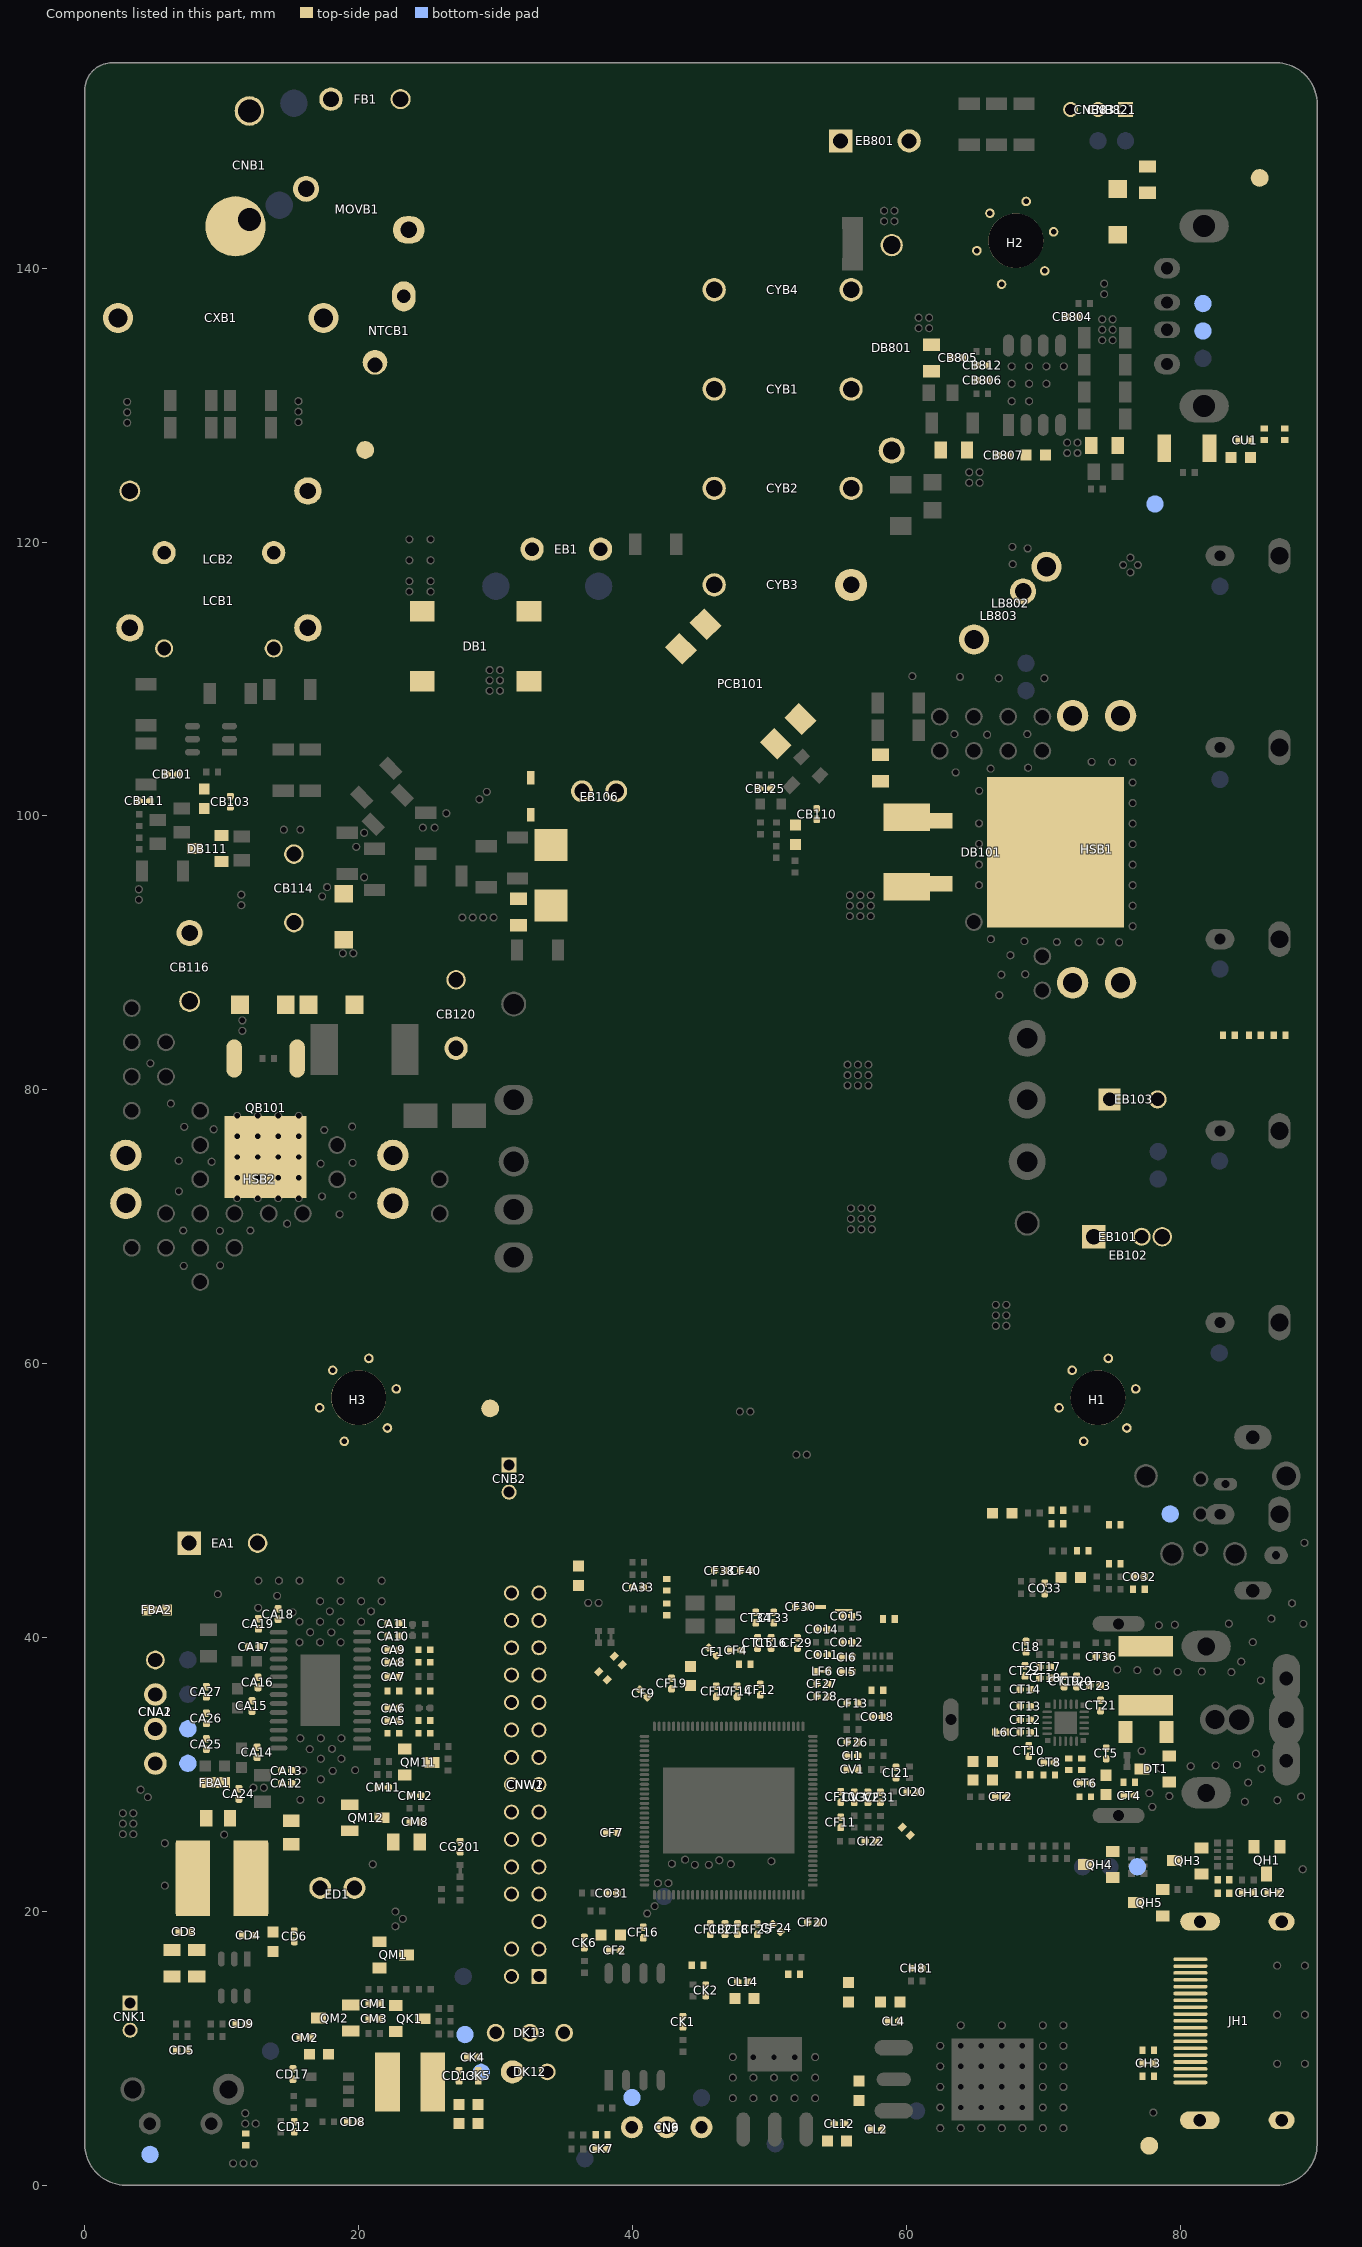
[diagram p0: the components of this part, seen from the top]
# Altium PCB MISC116569.PcbDoc (part 2 of 15)
Units mm, origin at the board's own origin, x right, y up, seen from the top; angles counter-clockwise.
Board outline 90 x 155 mm, 2 copper layers (TopLayer, BottomLayer), stack 1.571 mm thick; 527 components, 277 nets, 2450 pads, 649 vias.

## Components (designator, comment, footprint, x,y, rotation, side; value= is the part's Value field where it differs from the comment) (continued)
CA5 "0.22uF-0402-X5R-±10%-16V" C0402#1 22.539,33.929 r180 top
CA6 "0.22uF-0402-X5R-±10%-16V" C0402#1 22.539,34.849 r180 top
CA7 "1uF-0402-X5R-±20%-16V" C0402#1 22.539,37.145 r180 top
CA8 "1uF-0402-X5R-±20%-16V" C0402#1 22.539,38.177 r180 top
CA9 "NC/1uF-0402-X5R-±20%-16V" C0402#1 22.539,39.107 r180 top
CA10 "0.22uF-0402-X5R-±10%-16V" C0402#1 22.539,40.101 r180 top
CA11 "0.22uF-0402-X5R-±10%-16V" C0402#1 22.539,41.018 r180 top
CA12 "NC/0.1uF-0402-X5R-±20%-16V" C0402#1 14.752,29.358 r180 top
CA13 "1000pF-0402-X7R-±10%-50V" C0402#1 14.752,30.274 r180 top
CA14 "0.22uF-0402-X5R-±10%-16V" C0402#1 12.586,31.619 r270 top
CA15 "0.22uF-0402-X5R-±10%-16V" C0402#1 12.205,34.997 r270 top
CA16 "0.22uF-0402-X5R-±10%-16V" C0402#1 12.649,36.722 r90 top
CA17 "0.22uF-0402-X5R-±10%-16V" C0402#1 12.361,39.332 r180 top
CA18 "NC/0.1uF-0402-X5R-±20%-16V" C0402#1 14.122,41.716 r270 top
CA19 "1000pF-0402-X7R-±10%-50V" C0402#1 12.675,41.002 r270 top
CA24 "2200pF-0402-X7R-±10%-50V" C0402#1 11.252,28.581 r90 top
CA25 "2200pF-0402-X7R-±10%-50V" C0402#1 8.877,32.22 r90 top
CA26 "2200pF-0402-X7R-±10%-50V" C0402#1 8.877,34.095 r90 top
CA27 "2200pF-0402-X7R-±10%-50V" C0402#1 8.878,36.039 r270 top
CA31 "NC/10uF-0603-X5R-±20%-6.3V" C0603 67,49.075 r180 top
CA32 "NC/10uF-0603-X5R-±20%-6.3V" C0603 72.001,44.375 r180 top
CA33 "NC/1uF-0402-X5R-±20%-6.3V" C0402#1 40.411,43.665 r180 top
CAUTION "CAUTION" CAUTION 30.264,127.254 r180 bottom
CB101 "100pF-0402-NPO-±5%-50V" C0402#1 6.382,103.035 r180 top
CB102 "0.1uF-0603-X7R-±10%-50V" C0603 8.725,101.244 r270 top
CB103 "1000pF-0402-X7R-±10%-50V" C0402#1 10.63,101.041 r90 top
CB109 "Ceramic capacitor,CAP MC,25V,0.22uF,±10%,X7R,0603,SMD,TP" C0603 51.887,98.633 r270 top
CB110 "NC/1000pF-0402-X7R-±10%-50V" C0402#1 53.454,100.133 r90 top
CB111 "NC/Ceramic capacitor,CAP MC,50V,100pF,±5%,NPO,0402,SMD,TP" C0402#1 4.36,101.098 r0 top
CB113 "NC/220PF-0805-NPO-±10%-200V" C0805 31.661,92.989 r90 top
CB114 "Film capacitor,CAP PE,400V,4700pF,±5%,P,5.0mm,PC,DIP,TP,Fara" CAP8*2.5-V-5 15.269,94.709 r270 top locked
CB116 "Ceramic capacitor,CAP CD,2KV,100pF,±5%,SL,IK,5.0mm,DIP,TP,Walsin" CAP6.5*5-V-5-1 7.658,88.951 r270 top locked
CB118 "1000pF-0805-NPO-±10%-200V" C0805 58.11,103.505 r90 top
CB120 "NC/Ceramic capacitor,CAP CD,1KV,4700pF,±20%,Y5U,K,5.0mm,DIP,TP,Walsin" CAP10*4.5-V-5 27.114,85.534 r90 top locked
CB125 "NC/Ceramic capacitor,CAP MC,50V,0.022uF,±10%,X7R,0402,SMD,TP" C0402#1 49.677,101.994 r0 top
CB801 "Ceramic capacitor,CAP MC,25V,1uF,±10%,X7R,0603,SMD,TP" C0603 69.456,126.362 r180 top
CB804 "4700pF-0402-X7R-±10%-50V" C0402#1 72.098,136.449 r180 top
CB805 "NC/0.1uF-0402-X7R-±10%-16V" C0402#1 63.745,133.477 r180 top
CB806 "1000pF-0402-X7R-±10%-50V" C0402#1 65.54,131.826 r180 top
CB807 "100pF-0402-NPO-±5%-50V" C0402#1 67.076,126.34 r0 top
CB808 "220PF-0805-NPO-±10%-200V" C0805 77.597,146.468 r90 top
CB809 "220PF-0805-NPO-±10%-200V" C0805 74.481,127.051 r180 top
CB810 "220PF-0805-NPO-±10%-200V" C0805 63.469,126.733 r0 top
CB811 "220PF-0805-NPO-±10%-200V" C0805 61.831,133.452 r270 top
CB812 "0.033uF-0402-X7R-±10%-16V" C0402#1 65.54,132.918 r180 top
CD1 "NC/10uF-0805-X5R-±20%-16V" C0805 8.174,16.207 r270 top
CD2 "10uF-0805-X5R-±20%-16V" C0805 6.365,16.207 r270 top
CD3 "NC/0.1uF-0402-X5R-±20%-16V" C0402#1 7.276,18.504 r0 top
CD4 "Ceramic capacitor,CAP MC,16V,0.1uF,±10%,X7R,0402,SMD,TP" C0402#1 11.92,18.25 r0 top
CD5 "NC/56pF-0402-NPO-±5%-50V" C0402#1 7.088,9.868 r180 top
CD6 "NC/0.1uF-0402-X5R-±20%-16V" C0402#1 15.299,18.174 r90 top
CD7 "10uF-0603-X5R-±20%-6.3V" C0603 13.749,17.788 r90 top
CD8 "1uF-0402-X5R-±20%-6.3V" C0402#1 19.575,4.638 r180 top
CD9 "NC/0.1uF-0402-X5R-±20%-16V" C0402#1 11.434,11.786 r180 top
CD10 "NC/10uF-0603-X5R-±20%-6.3V" C0603 38.417,18.275 r180 top
CD12 "NC/NC/3300pF-0402-X7R-±10%-50V" C0402#1 15.299,4.27 r270 top
CD13 "NC/0.1uF-0402-X5R-±20%-16V" C0402#1 27.338,7.991 r270 top
CD14 "10uF-0603-X5R-±20%-6.3V" C0603 28.729,5.197 r90 top
CD15 "10uF-0603-X5R-±20%-6.3V" C0603 27.345,5.197 r90 top
CD16 "10uF-0603-X5R-±20%-6.3V" C0603 17.102,9.563 r180 top
CD17 "NC/0.1uF-0402-X5R-±20%-16V" C0402#1 15.197,8.118 r90 top
CF1 "Ceramic capacitor,CAP MC,50V,18pF,±5%,NPO,0402,SMD,TP" C0402#1 45.846,38.965 r315 top
CF2 "Ceramic capacitor,CAP MC,16V,0.1uF,±10%,X7R,0402,SMD,TP" C0402#1 38.714,17.147 r180 top
CF3 "10uF-0603-X5R-±20%-6.3V" C0603 44.221,37.186 r270 top
CF4 "Ceramic capacitor,CAP MC,50V,18pF,±5%,NPO,0402,SMD,TP" C0402#1 47.535,39.068 r180 top
CF5 "10uF-0603-X5R-±20%-6.3V" C0603 55.761,14.099 r90 top
CF7 "Ceramic capacitor,CAP MC,16V,0.1uF,±10%,X7R,0402,SMD,TP" C0402#1 38.482,25.745 r0 top
CF8 "Ceramic capacitor,CAP MC,16V,0.1uF,±10%,X7R,0402,SMD,TP" C0402#1 47.666,18.708 r90 top
CF9 "Ceramic capacitor,CAP MC,16V,0.1uF,±10%,X7R,0402,SMD,TP" C0402#1 40.8,35.918 r315 top
CF10 "Ceramic capacitor,CAP MC,16V,0.1uF,±10%,X7R,0402,SMD,TP" C0402#1 55.207,28.355 r90 top
CF11 "Ceramic capacitor,CAP MC,16V,0.1uF,±10%,X7R,0402,SMD,TP" C0402#1 55.207,26.505 r270 top
CF12 "Ceramic capacitor,CAP MC,16V,0.1uF,±10%,X7R,0402,SMD,TP" C0402#1 49.335,36.197 r270 top
CF13 "Ceramic capacitor,CAP MC,16V,0.1uF,±10%,X7R,0402,SMD,TP" C0402#1 56.071,35.204 r180 top
CF14 "Ceramic capacitor,CAP MC,16V,0.1uF,±10%,X7R,0402,SMD,TP" C0402#1 47.638,36.067 r270 top
CF15 "10uF-0603-X5R-±20%-6.3V" C0603 36.063,44.503 r270 top
CF16 "Ceramic capacitor,CAP MC,16V,0.1uF,±10%,X7R,0402,SMD,TP" C0402#1 40.787,18.456 r90 top
CF17 "Ceramic capacitor,CAP MC,16V,0.1uF,±10%,X7R,0402,SMD,TP" C0402#1 46.114,36.067 r270 top
CF18 "Ceramic capacitor,CAP MC,16V,0.1uF,±10%,X7R,0402,SMD,TP" C0402#1 45.683,18.708 r270 top
CF19 "Ceramic capacitor,CAP MC,16V,0.1uF,±10%,X7R,0402,SMD,TP" C0402#1 42.85,36.643 r90 top
CF20 "Ceramic capacitor,CAP MC,16V,0.1uF,±10%,X7R,0402,SMD,TP" C0402#1 53.187,19.192 r180 top
CF21 "1uF-0402-X5R-±20%-6.3V" C0402#1 46.749,18.708 r270 top
CF24 "1uF-0402-X5R-±20%-6.3V" C0402#1 50.525,18.792 r315 top
CF25 "1uF-0402-X5R-±20%-6.3V" C0402#1 49.112,18.708 r270 top
CF26 "0.047uF-0402-X7R-±10%-16V" C0402#1 56.07,32.36 r0 top
CF27 "NC/0.1uF-0402-X5R-±20%-16V" C0402#1 53.868,36.614 r180 top
CF28 "1uF-0402-X5R-±20%-6.3V" C0402#1 53.868,35.7 r180 top
CF29 "NC/1000pF-0402-X7R-±10%-50V" C0402#1 52.04,39.605 r270 top
CF30 "NC/1000pF-0402-X7R-±10%-50V" C0402#1 52.294,42.23 r0 top
CF31 "0.047uF-0402-X7R-±10%-16V" C0402#1 58.102,28.334 r270 top
CF38 "NC/30pF-0402-NPO-±5%-50V" C0402#1 46.375,44.884 r0 top
CF40 "Ceramic capacitor,CAP MC,50V,0.01uF,±10%,X7R,0402,SMD,TP" C0402#1 48.274,44.884 r180 top
CG201 "NC/0.1uF-0402-X5R-±20%-16V" C0402#1 27.414,24.719 r90 top
CH1 "NC/0.1uF-0402-X5R-±20%-16V" C0402#1 84.945,21.365 r0 top
CH2 "NC/0.1uF-0402-X5R-±20%-16V" C0402#1 86.8,21.364 r0 top
CH3 "NC/Ceramic capacitor,CAP MC,50V,22pF,±5%,NPO,0402,SMD,TP" C0402#1 77.664,8.905 r180 top
CH81 "1uF-0402-X5R-±20%-6.3V" C0402#1 60.765,15.839 r180 top
CI1 "0.047uF-0402-X7R-±10%-16V" C0402#1 56.062,31.355 r0 top
CI5 "Ceramic capacitor,CAP MC,16V,0.1uF,±10%,X7R,0402,SMD,TP" C0402#1 55.646,37.506 r0 top
CI6 "Ceramic capacitor,CAP MC,16V,0.1uF,±10%,X7R,0402,SMD,TP" C0402#1 55.646,38.572 r0 top
CI18 "NC/30pF-0402-NPO-±5%-50V" C0402#1 68.745,39.332 r270 top
CI20 "NC/NC/10pF-0402-NPO-±5%-50V" C0402#1 60.446,28.727 r0 top
CI21 "NC/NC/10pF-0402-NPO-±5%-50V" C0402#1 59.245,30.137 r270 top
CI22 "NC/NC/10pF-0402-NPO-±5%-50V" C0402#1 57.387,25.133 r0 top
CK1 "NC/0.1uF-0402-X7R-±20%-16V" C0402#1 43.683,11.937 r270 top
CK2 "Ceramic capacitor,CAP MC,50V,0.01uF,±10%,X7R,0402,SMD,TP" C0402#1 45.347,14.227 r270 top
CK4 "NC/0.1uF-0402-X5R-±20%-16V" C0402#1 28.341,9.362 r0 top
CK5 "NC/0.1uF-0402-X5R-±20%-16V" C0402#1 28.735,7.991 r270 top
CK6 "NC/10pF-0402-NPO-±5%-50V" C0402#1 36.482,17.719 r270 top
CK7 "NC/Ceramic capacitor,CAP MC,16V,0.1uF,±10%,X7R,0402,SMD,TP" C0402#1 37.731,2.657 r0 top
CL1 "NC/10uF-0603-X5R-±20%-6.3V" C0603 56.54,6.891 r270 top
CL2 "Ceramic capacitor,CAP MC,16V,0.1uF,±10%,X7R,0402,SMD,TP" C0402#1 57.818,4.079 r0 top
CL3 "NC/10uF-0603-X5R-±20%-6.3V" C0603 58.822,13.376 r0 top
CL4 "1uF-0402-X5R-±20%-6.3V" C0402#1 59.069,11.991 r0 top
CL11 "NC/10uF-0603-X5R-±20%-6.3V" C0603 54.935,3.241 r180 top
CL12 "Ceramic capacitor,CAP MC,16V,0.1uF,±10%,X7R,0402,SMD,TP" C0402#1 55.107,4.486 r180 top
CL13 "NC/10uF-0603-X5R-±20%-6.3V" C0603 48.179,13.642 r0 top
CL14 "1uF-0402-X5R-±20%-6.3V" C0402#1 48.056,14.861 r0 top
CM1 "Ceramic capacitor,CAP MC,16V,0.1uF,±10%,X7R,0402,SMD,TP" C0402#1 21.135,13.266 r180 top
CM2 "NC/0.1uF-0402-X5R-±20%-16V" C0402#1 16.112,10.782 r180 top
CM3 "NC/0.022uF-0402-X7R-±10%-16V" C0402#1 21.135,12.141 r180 top
CM7 "NC/10uF-0805-X5R-±20%-16V" C0805 23.489,25.07 r0 top
CM8 "NC/0.1uF-0402-X7R-±20%-16V" C0402#1 24.15,26.53 r180 top
CM11 "NC/0.1uF-0402-X5R-±20%-16V" C0402#1 21.783,29.046 r180 top
CM12 "0.022uF-0402-X7R-±10%-16V" C0402#1 24.15,28.448 r0 top
CN6 "NC/IR receiver,IR Receriver,2.5V~6V,38K,DIP,FDI-M6069560R538-WJGC25-D22,Fantasy" REMOTE-VD-9 42.494,4.177 r0 top locked
CN9 "IR receiver,IR Receriver,DIP,ARM-383AM1-Z-R-D10-22,ALL-BEST" REMOTE-VD-6 42.494,2.227 r0 top locked
CNA1 "Connector socket,connect jack,4Pin,D2.50,D,L=2.8mm,DIP,CNJST" SIP4/2.54D-1 5.156,34.575 r270 top locked
CNA2 "NC/4PIN-2.54-D-H-G-with latch-B" SIP4/2.5D-2 5.156,34.575 r270 top locked
CNB1 "连接插座,connect jack,2Pin,D7.92,L,SNAP,Fool-proofing,nature,L=2.8mm(11mm),DIP,A3962AW-3P2-A5WA-P-D(针长11.0mm),CNJST" CON2-H7.92 12.023,147.524 r0 top locked
CNB2 "Connector socket,connect jack,2Pin,D2.0,D,L=3.4mm,DIP,BOOM" SIP2/2.0D-1 30.988,51.61 r270 top
CNB821 "Connector socket,connect jack,2Pin,D2.0,D,L=3.4mm,DIP,BOOM" SIP2/2.0D-1 75.002,151.591 r180 top
CNB831 "Connector socket,connect jack,3Pin,D2.0,D,SNAP,L=2.8mm,DIP,CNJST" SIP3/2.0D-3 74.002,151.591 r180 top locked
CNK1 "NC/2PIN-2.0-D-H-G-LD" SIP2/2.0D-1 3.31,12.319 r270 top locked
CNW1 "Pin header,pin connector,2×15Pin/without pin6,D,D2.0mm,L=2.6mm,DIP,H2030-30SVB-V06-J8SY,XYDT" SIP2*15/2.0D-2 32.164,29.251 r270 top locked
CNW2 "NC/NC/连接插座,connect jack,2×15Pin/without pin6,D2.0,D,SNAP,Fool-proofing,Nature,L=2.6mm,DIP,CJ" SIP2*15/2.0D-11 32.164,29.251 r270 top locked
CO11 "NC/1000pF-0402-X7R-±10%-50V" C0402#1 53.835,38.735 r180 top
CO12 "NC/1uF-0402-X5R-±20%-6.3V" C0402#1 55.646,39.652 r0 top
CO14 "NC/1000pF-0402-X7R-±10%-50V" C0402#1 53.818,40.592 r180 top
CO15 "NC/1uF-0402-X5R-±20%-6.3V" C0402#1 55.646,41.557 r0 top
CO18 "NC/100pF-0402-X7R-±10%-50V" C0402#1 57.868,34.194 r180 top
CO31 "NC/NC/33pF-0402-NPO-±5%-50V" C0402#1 38.482,21.338 r180 top
CO32 "NC/Ceramic capacitor,CAP MC,16V,0.1uF,±10%,X7R,0402,SMD,TP" C0402#1 76.999,44.452 r0 top
CO33 "NC/330pF-0402-NPO-±5%-50V" C0402#1 70.104,43.587 r270 top
COLD "COLD" COLD 73.77,21.92 r90 top
"Conformal Coating" "NC/Conformal coating,25kg/Can,Peters" "Conformal Coating" 200.163,43.076 r90 top
CQC "CQC" CQC 18.712,39.029 r0 top
CT1 "10uF-0603-X5R-±20%-6.3V" C0603 65.583,29.581 r0 top
CT2 "NC/0.1uF-0402-X5R-±20%-16V" C0402#1 66.895,28.362 r180 top
CT3 "Ceramic capacitor,CAP MC,1KV,220pF,±5%,NPO,1206,SMD,TP" C1206 77.503,33.111 r0 top
CT4 "Thick-film resistor,RES,1/16W,0ohm,±1%,0402,SMD" C0402#1 76.271,28.45 r0 top
CT5 "NC/Ceramic capacitor,CAP MC,50V,120pF,±5%,NPO,0402,SMD,TP" C0402#1 74.595,31.537 r90 top
CT6 "Ceramic capacitor,CAP MC,50V,2pF,±0.25pF,NPO,0402,SMD,TP" C0402#1 73.065,29.365 r0 top
CT7 "Thick-film resistor,RES,1/16W,0ohm,±1%,0402,SMD" C0402#2 73.065,28.374 r0 top
CT8 "Ceramic capacitor,CAP MC,16V,0.1uF,±10%,X7R,0402,SMD,TP" C0402#1 70.44,30.875 r0 top
CT9 "Ceramic capacitor,CAP MC,50V,1000pF,±10%,X7R,0402,SMD,TP" C0402#2 70.441,29.96 r180 top
CT10 "Ceramic capacitor,CAP MC,16V,0.1uF,±10%,X7R,0402,SMD,TP" C0402#1 68.943,31.714 r270 top
CT11 "NC/Ceramic capacitor,CAP MC,50V,22pF,±5%,NPO,0402,SMD,TP,Walsin" C0402#1 68.683,33.079 r0 top
CT12 "NC/Ceramic capacitor,CAP MC,50V,27pF,±5%,NPO,0402,SMD,TP" C0402#1 68.683,33.988 r0 top
CT13 "NC/Ceramic capacitor,CAP MC,50V,22pF,±5%,NPO,0402,SMD,TP" C0402#1 68.683,34.978 r180 top
CT14 "NC/Ceramic capacitor,CAP MC,50V,22pF,±5%,NPO,0402,SMD,TP" C0402#1 68.689,36.21 r0 top
CT15 "Ceramic capacitor,CAP MC,16V,0.1uF,±10%,X7R,0402,SMD,TP" C0402#1 49.136,39.605 r270 top
CT16 "Ceramic capacitor,CAP MC,16V,0.1uF,±10%,X7R,0402,SMD,TP" C0402#1 50.127,39.605 r90 top
CT17 "NC/Ceramic capacitor,CAP MC,50V,1000pF,±10%,X7R,0402,SMD,TP" C0402#1 70.133,37.848 r0 top
CT18 "Ceramic capacitor,CAP MC,16V,0.1uF,±10%,X7R,0402,SMD,TP" C0402#1 70.133,37.046 r180 top
CT19 "Ceramic capacitor,CAP MC,50V,22pF,±5%,NPO,0402,SMD,TP" C0402#1 71.521,36.794 r270 top
CT20 "Ceramic capacitor,CAP MC,50V,22pF,±5%,NPO,0402,SMD,TP" C0402#1 72.436,36.794 r270 top
CT21 "Ceramic capacitor,CAP MC,16V,0.1uF,±10%,X7R,0402,SMD,TP" C0402#1 74.181,35.035 r90 top
CT22 "NC/0.1uF-0402-X5R-±20%-16V" C0402#1 68.664,37.565 r270 top
CT23 "NC/0.1uF-0402-X5R-±20%-16V" C0402#1 73.781,36.487 r0 top
CT33 "Ceramic capacitor,CAP MC,50V,18pF,±5%,NPO,0402,SMD,TP" C0402#1 50.31,41.456 r90 top
CT34 "Ceramic capacitor,CAP MC,50V,18pF,±5%,NPO,0402,SMD,TP" C0402#1 49.002,41.456 r270 top
CT36 "1uF-0402-X5R-±20%-6.3V" C0402#1 74.248,38.608 r180 top
CT52 "NC/10uF-0603-X5R-±20%-6.3V" C0603 65.583,30.952 r0 top
CU1 "1uF-0402-X5R-±20%-6.3V" C0402#1 84.698,127.419 r0 top
CU2 "NC/10uF-0603-X5R-±20%-6.3V" C0603 84.43,126.187 r0 top
CV1 "0.047uF-0402-X7R-±10%-16V" C0402#1 56.062,30.366 r180 top
CV2 "0.047uF-0402-X7R-±10%-16V" C0402#1 57.188,28.334 r90 top
CV3 "0.047uF-0402-X7R-±10%-16V" C0402#1 56.198,28.334 r90 top
CVBS_IN "DM0" TP 79.268,49.024 r180 bottom
CXB1 "X capacitor,CAP X2,MP,280VAC,0.47uF,±10%,S,15mm-Mini,PC,DIP,JH" CAP18*8.5-V-15 9.931,136.373 r180 top
CYB1 "Y capacitor,CAP Y1,CD,470pF,400VAC,±10%,KS,10mm,Y5P,DIP,Wansheng" CAP13*5-V-10-1#1 50.964,131.176 r0 top locked
CYB2 "Y capacitor,CAP Y1,CD,470pF,400VAC,±10%,KS,10mm,Y5P,DIP,Wansheng" CAP13*5-V-10-1#1 50.964,123.924 r0 top locked
CYB3 "Y capacitor,CAP Y1,CD,470pF,400VAC,±10%,KS,10mm,Y5P,DIP,Wansheng" CAP13*5-V-10-1#2 50.964,116.874 r0 top locked
CYB4 "Y capacitor,CAP Y1,CD,100pF,400VAC,±10%,K,10mm,Y5P,DIP,TP,TDK" CAP13*5-V-10-1#1 50.964,138.428 r0 top
D101 "NC/NC?" DIODE-S0402 51.798,15.42 r0 top
D102 "NC/NC?" DIODE-S0402 44.755,16.081 r0 top
DA31 "NC/NC?" DIODE-S0402 75.217,45.38 r180 top
DA32 "NC/NC?" DIODE-S0402 71.033,49.291 r0 top
DA33 "NC/NC?" DIODE-S0402 72.88,46.319 r180 top
DAS1 "35.0*5.4mm" DOLBY_AS2 75.298,14.948 r180 top
DB1 "Bridge rectifier,DIO BRD,3A,800V,YBS,SMD,YBS3010A,YJ" B/YBS3010A 28.545,112.395 r270 top
DB101 "Schottky diode,DIO SBD D1,10A,150V,TO-263,SMD,HBR10150SS,JLHW" D2PAK3 67.528,97.457 r180 top
DB104 "Rectifier diode,DIO SI S,1A,1000V,SMAF,SMD,M7F,YJ" DIODE-S-1 34.05,95.658 r90 top
DB106 "Rectifier diode,DIO FRD S,1.2A,800V,eSGA,SMD,R12K,GOOD-ARK" DIODE-S-14 18.898,92.635 r270 top
DB109 "Rectifier diode,DIO FRD S,1.2A,800V,SOD-123FL,SMD,F1K,YJ" DIODE-S-14 13.006,86.198 r180 top
DB110 "Rectifier diode,DIO FRD S,1.2A,800V,SOD-123FL,SMD,F1K,YJ" DIODE-S-14 18.021,86.198 r180 top
DB111 "Switching diode,DIO SW D1,215mA,85V,SOT-23,SMD,KAV70,KEXIN" SO-23 8.966,97.612 r270 top
DB121 "NC/BAV21WS" DIODE-S-12 32.563,101.439 r270 top
DB801 "Schottky diode,DIO SBD S,2A,100V,DO-15,DIP,SR2100,YJ" D2-H-15 58.929,134.186 r90 top locked
DB804 "Rectifier diode,DIO FRD S,1.2A,800V,SOD-123FL,SMD,F1K,YJ" DIODE-S-14 75.433,144.12 r90 top
DBS8 "DOLBY Double-D" Double-D-SILK 84.148,97.163 r180 bottom
DH1 "NC/Ceramic capacitor,CAP MC,50V,22pF,±5%,NPO,0402,SMD,TP" DIODE-S0402 77.668,9.845 r180 top
DH2 "NC/SFI0402-240E-2R5PP-LF" DIODE-S0402 83.161,21.338 r180 top
DH3 "NC/SFI0402-240E-2R5PP-LF" DIODE-S0402 83.161,22.304 r180 top
DH81 "NC/SFI0402-240E-2R5PP-LF" DIODE-S0402 77.668,7.965 r180 top
DI1 "NC/AIES12U020R2" DIODE-S0402 71.033,48.313 r0 top
DI2 "NC/AIES12U020R2" DIODE-S0402 76.988,43.513 r180 top
DI3 "NC/AIES12U020R2" DIODE-S0402 75.217,48.224 r180 top
DI10 "NC/AVLC18S02003" DIODE-S0402 42.489,42.052 r90 top
DI11 "NC/AVLC18S02003" DIODE-S0402 42.489,43.856 r90 top
DK1 "NC/AVLC18S02003" DIODE-S0402 11.768,3.34 r270 top
DK3 "NC/AVLC18S02003" DIODE-S0402 37.739,3.673 r180 top
DK12 "NC/Light-emitting diode,Single LED,RED,25mA,28mcd,638nm,1.9V,φ3.85×5.4mm,DIP,HL" LED-HD-6 32.505,5.624 r0 top locked
DK13 "Light-emitting diode,Double LED,R/G,30mA,700/450mcd,625/570nm,2.1/2.1V,Φ3×5.3mm,DIP,WEJ3290C-R3H8-BC,WEJ" LED-HD-5 32.505,11.127 r0 top locked
DM0 "DM0" TP 81.656,135.417 r180 bottom
DP0 "DM0" TP 81.656,137.417 r180 bottom
DT1 "Switching diode,DIO SW D2,200mA,100V,SOT-23,SMD,BAV99,YJ" SO-23 78.176,30.406 r270 top
DU1 "NC/Thick-film resistor,TVS diode,DIO ESD,0.1pF,25V,0402,SMD,GESD1005H150CR10GPT,Sunlord" DIODE-S0402 87.625,127.876 r90 top
DU2 "NC/Thick-film resistor,TVS diode,DIO ESD,0.1pF,25V,0402,SMD,GESD1005H150CR10GPT,Sunlord" DIODE-S0402 86.126,127.876 r90 top
DU3 "NC/Thick-film resistor,TVS diode,DIO ESD,0.1pF,25V,0402,SMD,GESD1005H150CR10GPT,Sunlord" DIODE-S0402 38.959,38.318 r135 top
DU4 "NC/Thick-film resistor,TVS diode,DIO ESD,0.1pF,25V,0402,SMD,GESD1005H150CR10GPT,Sunlord" DIODE-S0402 37.841,37.213 r315 top
DV3 "NC/AVLC18S02003" DIODE-S0402 85.453,83.988 r180 top
DV4 "NC/AVLC18S02003" DIODE-S0402 83.555,83.988 r0 top
DV5 "NC/AVLC18S02003" DIODE-S0402 87.257,83.988 r180 top
DV7 "NC/AVLC18S02003" DIODE-S0402 57.887,36.144 r0 top
DV8 "NC/AVLC18S02003" DIODE-S0402 58.731,41.351 r180 top
DV9 "NC/AVLC18S02003" DIODE-S0402 59.986,25.853 r315 top
EA1 "Aluminum electrolytic capacitor,CAP AL,16V,470uF,±20%,PKRM,P,5.0mm,10×12.5,DIP,TP,Koshin" EC(10*12)-V-5 10.123,46.888 r0 top locked
EB1 "Aluminum electrolytic capacitor,CAP AL,400V,47uF,±20%,KY,BW,5.0mm,13×30,DIP,CapXon" EC(13*30)-H-5 35.166,119.484 r180 top locked
EB101 "Aluminum electrolytic capacitor,CAP AL,16V,270uF,±20%,SP,RP,S,3.5mm,8×11,DIP,Elite" EC(8*11)-V-3.5 75.437,69.266 r0 top
EB102 "Aluminum electrolytic capacitor,CAP AL,25V,470uF,±20%,LD,PKLH,P,5.0mm,10×12.5,DIP,TP,Koshin" EC(10*12.5)-V-5#1 76.187,69.266 r0 top locked
EB103 "Aluminum electrolytic capacitor,CAP AL,16V,270uF,±20%,SP,RP,S,3.5mm,8×11,DIP,Elite" EC(8*11)-V-3.5 76.599,79.299 r0 top
EB106 "Aluminum electrolytic capacitor,CAP AL,50V,10uF,±20%,LF,PKZF,P,2.5mm,5×11,DIP,TP,Koshin" EC(5*11)-V-2.5 37.561,101.803 r0 top locked
EB801 "Aluminum electrolytic capacitor,CAP AL,100V,47uF,±20%,LD,PKLW,P,5.0mm,10×12.5,DIP,TP,Koshin" EC(10*12.5)-V-5#2 57.704,149.299 r0 top locked
ED1 "Aluminum electrolytic capacitor,CAP AL,10V,470uF,±20%,PKZH,P,2.5mm,6.3×11,DIP,TP,Koshin" EC(6.3*11)-V-2.5 18.443,21.707 r0 top
EVA1 "NC/7×7×3mm-C-4305 fire-retardant foam-Black" EVA(7*7*3) 42.291,54.013 r180 bottom
EVA2 "NC/7×7×3mm-C-4305 fire-retardant foam-Black" EVA(7*7*3) 85.268,111.239 r180 bottom
EVA3 "NC/7×7×3mm-C-4305 fire-retardant foam-Black" EVA(7*7*3) 34.519,147.193 r180 bottom
EVA4 "NC/7×7×3mm-C-4305 fire-retardant foam-Black" EVA(7*7*3) 10.693,75.286 r180 bottom
FB1 "Slow-blow fuse,FUSE T,P,3.15A,250VAC,8.5×4.0×8mm,DIP,TP,Walter" "FUSE8.5*4-V-5(T3.15AL 250V~)" 20.52,152.348 r180 top locked
FBA1 "NC/0ohm-0603-PCB" R0603SC#1 9.481,29.401 r180 top
FBA2 "NC/0ohm-0603-PCB" R0603SC#2 5.271,42.024 r180 top
FT2 "Ferrite bead,BEAD,1000ohm,0402,300mA,SMD,TRAY,CBM100505U102T,FH" L0402 68.62,29.962 r180 top
FU1 "NC/NSMD110(1206-1.1A)" FUSE1.1A-S 80.488,126.848 r180 top
GD1 "7.00×8.35mm-Nylon-White-WQM" Fixed 55.5,97 r0 top
GD2 "7.00×8.35mm-Nylon-White-WQM" Fixed 46,150.5 r0 top locked
GD3 "7.00×8.35mm-Nylon-White-WQM" Fixed 4.5,53 r0 top locked
GDT1 "NC/Gas discharge tube,GDT,700V,2000A,TP,4.5×3.2mm,SMD,4532-091-LF,Brightking" SMD4532-1 77.478,37.201 r90 top
GL1 "Silicone,0.5g,general purpose,60,White,SLD-8854W,XY" "Silica gel-15" 35.293,140.919 r180 top
GL3 "Silicone,0.5g,general purpose,60,White,SLD-8854W,XY" "Silica gel-5*3" 44.468,4.964 r0 top
GL4 "Silicone,0.5g,general purpose,60,White,SLD-8854W,XY" "Silica gel-5*3" 32.982,7.468 r0 top
GL5 "NC/Silicone,0.5g,general purpose,60,White,SLD-8854W,XY" "Silica gel-10" 57.823,114.605 r180 top
GL6 "NC/Silicone,0.5g,general purpose,60,White,SLD-8854W,XY" "Silica gel-10" 45.225,136.081 r0 top
GL7 "NC/Silicone,0.5g,general purpose,60,White,SLD-8854W,XY" "Silica gel-10" 45.005,130.834 r0 top
GL8 "NC/Silicone,0.5g,general purpose,60,White,SLD-8854W,XY" "Silica gel-10" 45.25,127.749 r0 top
GND "" TP 76.873,23.254 r180 bottom
H1 "Location hole" ASSE4.0C-3 74,57.502 r0 top locked
H2 "Location hole" ASSE4.0C-3 68,142.004 r0 top locked
H3 "Location hole" ASSE4.0C-3 20,57.502 r0 top locked
"High Voltage" "High Voltage" "High Voltage" 26.352,147.307 r90 top
HOT "HOT" HOT 33.083,110.122 r90 top
HS1 "NC/Heat sink,15.0×15.0×5.0mm,AL1060H-24,Black,high-emissivity paint spray,stamped with bends,no rivet pins,YT" HS(15X15X5)-S 47.025,27.357 r90 top locked
HSB1 "NC/Heat sink,17.5×14.5×0.5mm,copper sheet,matte tin plated,natural color,four pins,WT" HS151-TEMP-NG 73.891,97.571 r90 top
HSB2 "NC/Heat sink,17.5×14.5×0.5mm,copper sheet,matte tin plated,natural color,four pins,WT" HS151-TEMP-NG 12.754,73.459 r180 top locked
IR_IN "TEST  SL" TP 39.962,6.403 r180 bottom
JH1 "HDMI jack,HDMI Jack,H,SMD,161031041(hull-SPCC ),VAST" HDMI-HS-1 91.999,12 r90 top locked
K0 "TEST  SL" TP 4.77,2.25 r180 bottom
L3 "Thick-film resistor,RES,1/16W,0ohm,±1%,0402,SMD" L0402 48.192,38.052 r180 top
L6 "NC/0ohm-0402-PCB" R0402SC#1 66.899,33.086 r0 top
LB802 "Differential-mode inductor,Inductor,DR12×12,70uH,0.15×12P,38.5Ts,H13.5MAX,SYDR1212-L070uA,DIP,EDL" L/LC2/15*14.5-V7.5 67.592,115.545 r45 top
LB803 "NC/Differential-mode inductor,Inductor,DR12×14,68uH,0.45,20Ts,H13.5MAX,SYDR1214-L068uA,DIP,Soldier" L(13.5*15.5)-V-5 66.761,114.633 r45 top
LCB1 "共模电感,Common Choke,UU9.8,20mH MIN,0.27×1P,86Ts,H14.0MAX,SYUU9.8-L002,DIP,CK" L/LC4/UU9.8/7*8-H 9.793,115.731 r180 top
LCB2 "NC/SYUU10.5-L002-JM" L/UU10.5/10*13-2 9.793,118.731 r90 top
LD1 "Power inductor,Power Inductor,4.7uH,±20%,2.8A,0.32×1P,DR5.8×4.5,SMD,PIO54-4R7MTP02,FH" L(5.8*4.5)-S 10.013,22.424 r180 top
LD2 "Power inductor,Power Inductor,2.2uH,±20%,2A,0.28×1P,DR4.5×3.2,SMD,PIO43-2R2MTP02,FH" L(4.5*3.5)-S 23.757,7.527 r180 top
LD3 "NC/Power inductor,Power Inductor,4.7uH,±20%,3.3A,DR6.0×4.5,SMD,SWPA6045S4R7MT,Sunlord" L(6.0*4.5)-S 10.007,22.424 r180 top
LED_G "TEST  SL" TP 27.764,11.001 r180 bottom
LED_R "TEST  SL" TP 28.951,8.245 r180 bottom
LF6 "NC/0ohm-0402-PCB" R0402SC#1 53.867,37.519 r180 top
LOUT+ "DM0" TP 7.526,30.811 r180 bottom
LOUT- "DM0" TP 7.526,33.331 r180 bottom
LT1 "NC/Multilayer inductor,HF Inductor,330nH,±5%,0402,SMD,SDCL1005CR33JTDF,Sunlord" L0402 76.284,29.416 r0 top
LT2 "NC/Multilayer inductor,HF Inductor,270nH,±5%,0603,SMD,HCI1608F-R27J-M,Tai-tech" L0603 74.595,29.238 r90 top
LT3 "Multilayer inductor,HF Inductor,6.8nH,±5%,0402,SMD,MGCI1005T6N8JT-LF,Sunlord" L0402 72.817,30.749 r90 top
LT4 "Ferrite bead,BEAD,1000ohm,0402,300mA,SMD,TRAY,CBM100505U102T,FH" L0402 71.852,30.749 r90 top
M1 "MARK" MARK 20.475,126.729 r0 top (schematic designator M4)
M2 "MARK" MARK 77.737,2.883 r0 top
M3 "MARK" MARK 85.801,146.596 r0 top
M4 "MARK" MARK 29.604,56.731 r0 top
Manufacture_Info "Manufacture_Info" MANUFACTURE_INFO 19.387,29.134 r180 top
ML1 "NC/Latest Mylar sheet" Mylar 163.512,74.295 r90 top
MOVB1 "NC/Varistor,VARISTOR,128J,680V,4000A,S,7.5mm,10mm,DIP,Thinking" VR(13*5)-V-7.5 19.909,144.297 r0 top
NTCB1 "NTC thermistor,RES NTC,2.4W,5A,2.5ohm,±20%,S,5.0mm,10mm,DIP,FH" NTC(10*5)-V5 22.244,135.447 r90 top
PCB101 "LTV-817S-TA-B (Lite-On)" OC4-S-1 47.9,109.639 r45 top
PWM_REF "NC/TEST" TP_BL 78.156,122.784 r270 bottom
QB101 "MOSFET,NMOS,5A,650V,0.8ohm@ID=2.5A@VGS=10V,TO-252,SVS5N70D,SL" TO-252-GDS 13.207,75.083 r180 top
QH1 "General-purpose transistor,Dynatron,NPN,0.2A,40V,30-300,SOT-23,LMBT3904LT1G,LRC" SOT-23 86.33,23.701 r0 top
QH3 "General-purpose transistor,Dynatron,NPN,0.2A,40V,30-300,SOT-23,LMBT3904LT1G,LRC" SOT-23 80.538,23.688 r270 top
QH4 "General-purpose transistor,Dynatron,NPN,0.2A,40V,30-300,SOT-23,LMBT3904LT1G,LRC" SOT-23 74.066,23.419 r270 top
QH5 "General-purpose transistor,Dynatron,NPN,0.2A,40V,30-300,SOT-23,LMBT3904LT1G,LRC" SOT-23 77.719,20.627 r270 top
QK1 "General-purpose transistor,Dynatron,NPN,0.2A,40V,30-300,SOT-23,LMBT3904LT1G,LRC" SOT-23 23.731,12.169 r90 top
QM1 "General-purpose transistor,Dynatron,NPN,0.2A,40V,30-300,SOT-23,LMBT3904LT1G,LRC" SOT-23 22.538,16.828 r90 top
QM2 "MOSFET,PMOS,-4.4A,-30V,0.046ohm@ID=-4A@VGS=-4.5V,SOT-23,NCE3401AY,NCEPOWER" SOT-23-1 18.22,12.205 r270 top
QM11 "General-purpose transistor,Dynatron,NPN,0.2A,40V,30-300,SOT-23,LMBT3904LT1G,LRC" SOT-23 24.379,30.899 r90 top
QM12 "MOSFET,PMOS,-4.3A,-30V,0.048ohm@ID=-3A@VGS=-4.5V,SOT-23-3L,NCE3407AY,NCEPOWER" SOT-23-1 20.556,26.835 r90 top
R5V "NC/Thick-film resistor,RES,1/8W,0ohm,±1%,0805,SMD" R0805 15.07,25.756 r90 top
R12V "Thick-film resistor,RES,1/8W,0ohm,±1%,0805,SMD" R0805 9.738,26.81 r0 top
RA1 "4K7ohm-0402-±1%-1/16W" R0402 24.804,33.011 r0 top
RA2 "4K7ohm-0402-±1%-1/16W" R0402 22.539,33.011 r0 top
RA3 "1Kohm-0402-±1%-1/16W" R0402 24.804,33.929 r180 top
RA4 "NC/?" GND#1 55.425,41.997 r180 top
RA5 "NC/?" GND#2 53.465,42.23 r180 top
RA8 "NC/100Kohm-0402-±5%-1/16W" R0402 22.539,36.087 r180 top
RA9 "NC/47Kohm-0402-±5%-1/16W" R0402 24.804,36.087 r180 top
RA10 "10Kohm-0402-±1%-1/16W" R0402 24.804,38.195 r0 top
RA11 "NC/15Kohm-0402-±1%-1/16W" R0402 24.804,39.107 r0 top